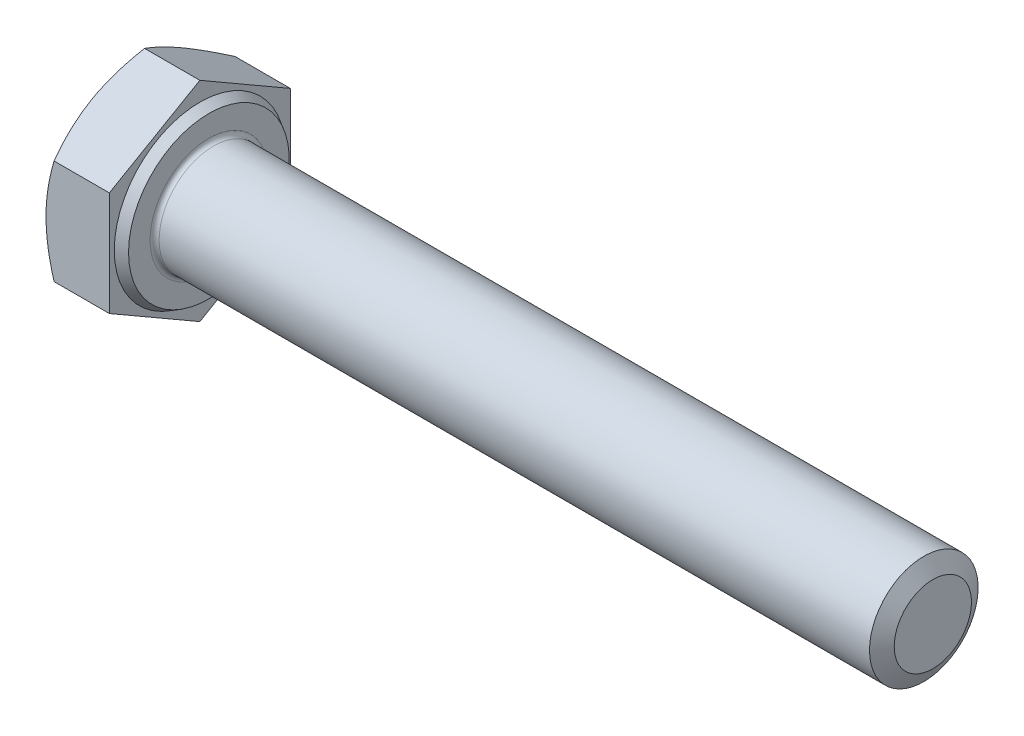
SolidWorks part; units mm, degrees
ref_plane "前视" through (0, 0, 0) normal (0, 0, 1) x (1, 0, 0)
ref_plane "上视" through (0, 0, 0) normal (0, 1, 0) x (1, 0, 0)
ref_plane "右视" through (0, 0, 0) normal (1, 0, 0) x (0, 0, -1)
sketch "草图1" plane through (0, 0, 0) normal (1, 0, 0) x (0, 0, -1)
  line L0 (5, 2.8868) -> (5, -2.8868)
  line L1 (-5, 2.8868) -> (-5, -2.8868)
  line L2 (5, -2.8868) -> (0, -5.7735)
  line L3 (0, -5.7735) -> (-5, -2.8868)
  line L4 (5, 2.8868) -> (0, 5.7735)
  line L5 (0, 5.7735) -> (-5, 2.8868)
  circle A0 centre (0, 0) radius 5.525 construction
  dimension "e" = 11.05
  dimension "s" = 10
  dimension "D2" = 120
  dimension "D3" = 5
  dimension "D4" = 5
  dimension "D5" = 5
extrude "基体-拉伸" add sketch "草图1" along normal blind 4
sketch "草图2" plane through (0, 0, 0) normal (0, 0, 1) x (1, 0, 0)
  line L0 (0, 2.8868) -> (0, -2.8868) construction
  line L1 (0, 0) -> (44, 0)
  line L2 (0, 0) -> (0, 3)
  line L3 (0, 3) -> (44, 3)
  line L4 (44, 0) -> (44, 2.134)
  line L5 (4, 5.7735) -> (4, 2.8868) construction
  line L6 (0, 0) -> (-6.8, 0) construction
  line L7 (0, 0) -> (22, 0) construction
  line L8 (44, -2.134) -> (90.335, -3) construction
  line L9 (0, -3) -> (90.335, -3) construction
  line L10 (5, 3) -> (5, 0) construction
  line L11 (4, 13.0554) -> (4, -1.27) construction
  line L12 (4, 2.8868) -> (4, -2.8868) construction
  line L14 (44, 3) -> (44, 2.134)
  dimension "l" = 40
  dimension "d" = 6
  dimension "Minor_dia" = 4.268
  dimension "p" = 1
  dimension "b" = 40
  dimension "da" = 6.8
revolve "凸台-旋转1" add sketch "草图2" angle 360 about L7
cosmetic thread "螺旋线1" parameters "Thread_length"=39, "Thread_minor"=4.268
sketch "草图3" plane through (0, 0, 0) normal (0, 0, 1) x (1, 0, 0)
  line L0 (0, 5) -> (3.3333, 10.7735)
  line L1 (0, 5.7735) -> (0, 2.8868) construction
  line L2 (3.3333, 10.7735) -> (3.3333, 15.7735)
  line L3 (3.3333, 15.7735) -> (-10, 15.7735)
  line L4 (-10, 15.7735) -> (-10, 5)
  line L5 (-10, 5) -> (0, 5)
  line L6 (0, 0) -> (99.06, 0) construction
  line L7 (4, 5.7735) -> (0, 5.7735) construction
  dimension "D1" = 5
  dimension "D2" = 5
  dimension "D3" = 10
  dimension "D4" = 5
  dimension "Head_ch_ang" = 30
revolve "切除-旋转1" cut sketch "草图3" angle 360 about L6
sketch "草图4" plane through (0, 0, 0) normal (0, 0, 1) x (1, 0, 0)
  line L0 (0, 0) -> (248.9073, 0) construction
  line L2 (4, 0) -> (4, 4.44) construction
  line L3 (4, -3) -> (4, 3) construction
  line L4 (4, 5.7735) -> (4, 2.8868) construction
  line L9 (4, 4.44) -> (3.5, 4.7287)
  line L10 (3.5, 4.7287) -> (3.5, 5.7735)
  line L11 (4, 5.7735) -> (0.4466, 5.7735) construction
  line L12 (3.5, 5.7735) -> (4, 5.7735)
  line L13 (4, 5.7735) -> (4, 4.44)
  dimension "D1" = 120
  dimension "c" = 0.5
  dimension "dw" = 8.88
revolve "切除-旋转3" cut sketch "草图4" angle 360 about L0
fillet "圆角" radius 0.25 1 edges at (4, 0, -3)
sketch "草图6" plane through (0, 0, 0) normal (0, 0, 1) x (1, 0, 0)
  line L0 (0, 0) -> (44, 0) construction
  line L1 (44, -3) -> (44, 3) construction
  line L2 (44, 0) -> (44, 3) construction
  line L4 (43.5, 3) -> (44.5, 3)
  line L5 (43.5, 3) -> (44, 2.134)
  line L6 (44, 2.134) -> (44.5, 3)
  dimension "D1" = 1
revolve "切除-旋转4" cut sketch "草图6" angle 360 about L0
pattern_linear "阵列(线性)1" [suppressed]
